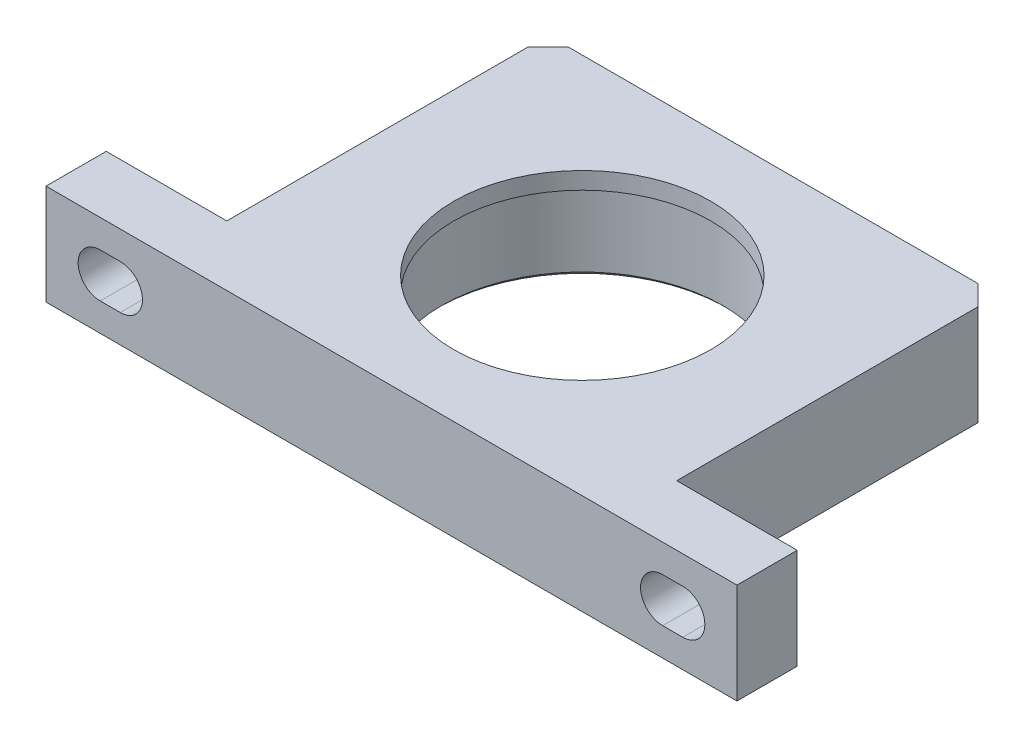
SolidWorks part; units mm, degrees
material "普通碳钢"
ref_plane "Front Plane" through (0, 0, 0) normal (0, 0, 1) x (1, 0, 0)
ref_plane "Top Plane" through (0, 0, 0) normal (0, 1, 0) x (1, 0, 0)
ref_plane "Right Plane" through (0, 0, 0) normal (1, 0, 0) x (0, 0, -1)
other "Configuration Table"
sketch "Sketch1" plane through (0, 0, 0) normal (0, 1, 0) x (1, 0, 0)
  line L0 (-172, 0) -> (172, 0)
  line L1 (-172, 0) -> (-172, 30)
  line L2 (-172, 30) -> (-112, 30)
  line L3 (172, 0) -> (172, 30)
  line L4 (172, 30) -> (112, 30)
  line L5 (-112, 30) -> (-91.4684, 116.6686)
  line L6 (0, 0) -> (0, 189) construction
  line L7 (91.4684, 116.6686) -> (112, 30)
  arc A0 (91.4684, 116.6686) -> (-91.4684, 116.6686) centre (0, 95) ccw
  circle A1 centre (0, 95) radius 64
  point P4 (0, 0)
  point P11 (0, 125.759)
  dimension "D7" = 188
  dimension "D9" = 128
  dimension "D1" = 344
  dimension "D2" = 30
  dimension "D3" = 60
  dimension "D4" = 30
  dimension "D5" = 60
  dimension "D6" = 189
  dimension "D8" = 95
extrude "Boss-Extrude1" add sketch "Sketch1" along normal mid plane 50
sketch "Sketch2" plane through (0, -25, 0) normal (0, -1, 0) x (1, 0, 0)
  circle A0 centre (0, -95) radius 70
  dimension "D1" = 140
extrude "Cut-Extrude1" cut sketch "Sketch2" against normal blind 41.5
chamfer "Chamfer1" distance 2 angle 45 1 edges at (0, -25, -165)
fillet "Fillet1" radius 2 1 edges at (0, 16.5, -165)
sketch "Sketch3" plane through (0, 0, -30) normal (0, 0, -1) x (-1, 0, 0)
  line L0 (135, 0) -> (145, 0) construction
  line L1 (135, 11) -> (145, 11)
  line L2 (135, -11) -> (145, -11)
  line L3 (-145, 0) -> (-135, 0) construction
  line L4 (-145, 11) -> (-135, 11)
  line L5 (-145, -11) -> (-135, -11)
  line L6 (-172, 25) -> (-112, 25) construction
  arc A0 (135, 11) -> (135, -11) centre (135, 0) ccw
  arc A1 (145, -11) -> (145, 11) centre (145, 0) ccw
  arc A2 (-145, 11) -> (-145, -11) centre (-145, 0) ccw
  arc A3 (-135, -11) -> (-135, 11) centre (-135, 0) ccw
  point P2 (140, 0)
  point P7 (-140, 0)
  dimension "D1" = 280
  dimension "D2" = 22
  dimension "D3" = 22
  dimension "D4" = 10
  dimension "D5" = 10
  dimension "D6" = 140
  dimension "D7" = 25
extrude "Cut-Extrude2" cut sketch "Sketch3" against normal blind 41.5
sketch "Sketch4" plane through (0, -25, 0) normal (0, -1, 0) x (1, 0, 0)
  line L0 (-112, -30) -> (-112, -190)
  line L1 (-112, -190) -> (112, -190)
  line L2 (112, -30) -> (112, -190)
  line L3 (112, -30) -> (91.4684, -116.6686) construction
  line L4 (-91.4684, -116.6686) -> (-112, -30) construction
  line L5 (112, -30) -> (91.4684, -116.6686)
  line L6 (-91.4684, -116.6686) -> (-112, -30)
  arc A2 (-91.4684, -116.6686) -> (91.4684, -116.6686) centre (0, -95) ccw construction
  arc A3 (-91.4684, -116.6686) -> (91.4684, -116.6686) centre (0, -95) ccw
  point P6 (0, -194.8364)
  dimension "D1" = 160
extrude "Boss-Extrude2" add sketch "Sketch4" against normal blind 50
chamfer "Chamfer2" distance 10 angle 45 2 edges at (-112, 0, -190) (112, 0, -190)
